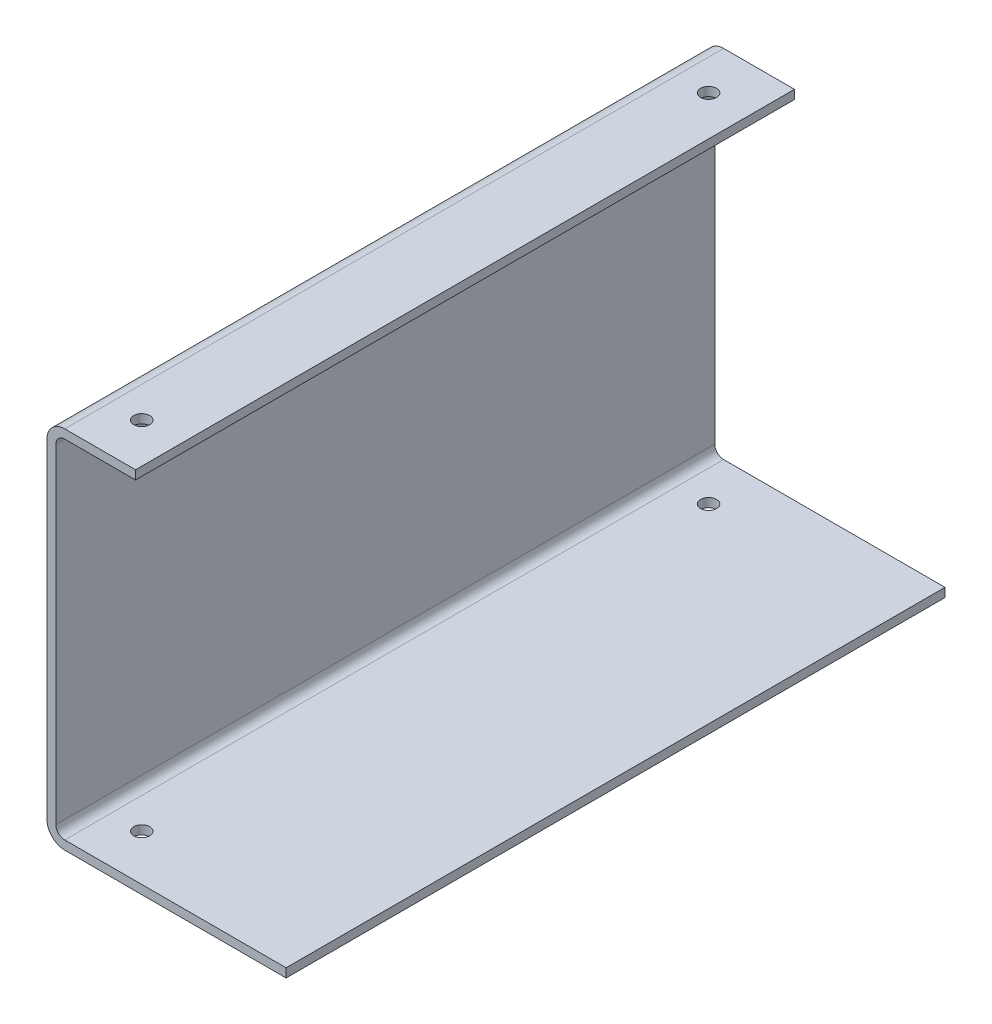
from build123d import *

# Parameters (mm, degrees)
EXTRUDE_THIN1_DEPTH = 372
SKETCH2_R           = 4.5
CUT_EXTRUDE1_DEPTH  = 447.144595395
LPATTERN1_COUNT     = 2
LPATTERN1_PITCH     = 320


with BuildPart() as part:
    # Sketch1 → Extrude-Thin1 (new body)
    with BuildSketch(Plane.XY):
        with BuildLine():
            Line((50, 206), (10, 206))
            ThreePointArc((10, 206), (2.928932188, 203.071067812), (0, 196))
            Line((0, 196), (0, 10))
            ThreePointArc((0, 10), (2.928932188, 2.928932188), (10, 0))
            Line((10, 0), (135, 0))
            Line((135, 0), (135, 5))
            Line((135, 5), (10, 5))
            ThreePointArc((10, 5), (6.464466094, 6.464466094), (5, 10))
            Line((5, 10), (5, 196))
            ThreePointArc((5, 196), (6.464466094, 199.535533906), (10, 201))
            Line((10, 201), (50, 201))
            Line((50, 201), (50, 206))
        make_face()
    extrude(amount=EXTRUDE_THIN1_DEPTH)

    # Sketch2 → Cut-Extrude1 (cut, through all)
    with BuildSketch(Plane(origin=(0, 206, 0), x_dir=(1, 0, 0), z_dir=(0, 1, 0))):
        with Locations(Location((27.5, -346, 0), (0, 0, 270))):
            Circle(SKETCH2_R)
    cut_extrude1 = extrude(amount=-CUT_EXTRUDE1_DEPTH, mode=Mode.SUBTRACT)

    # LPattern1: Cut-Extrude1 ×2
    with Locations(*[(0, 0, -i * LPATTERN1_PITCH) for i in range(1, LPATTERN1_COUNT)]):
        add(cut_extrude1, mode=Mode.SUBTRACT)


solid = part.part
